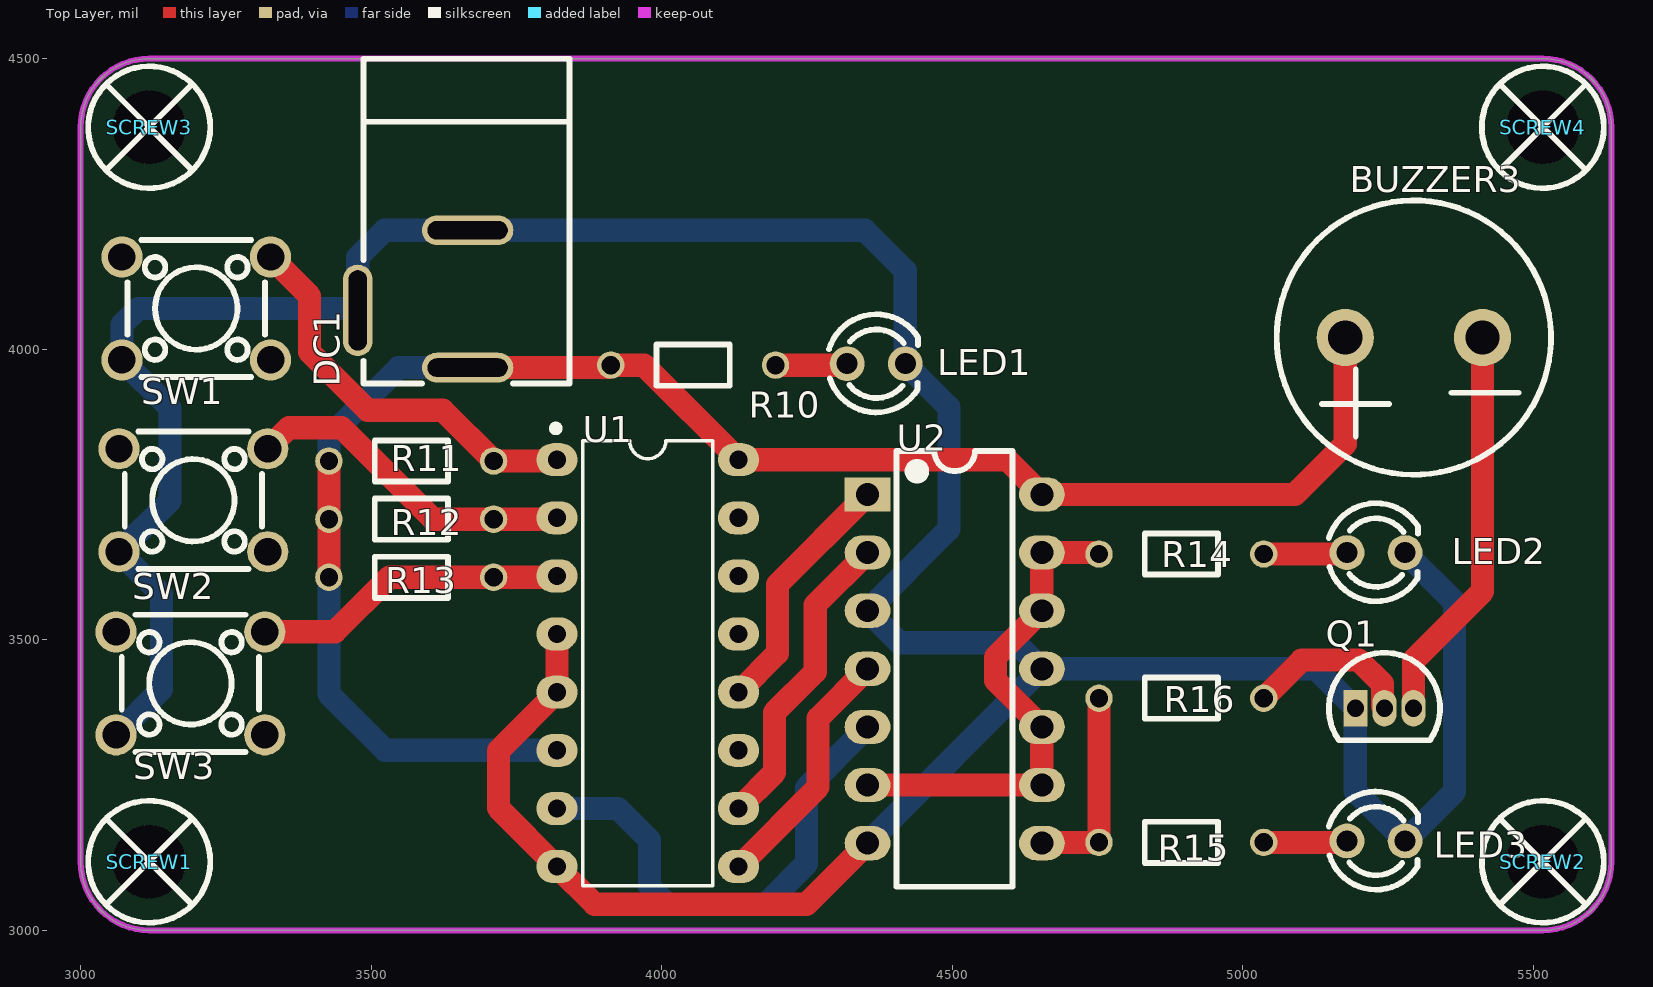
[diagram p0: Top Layer view]
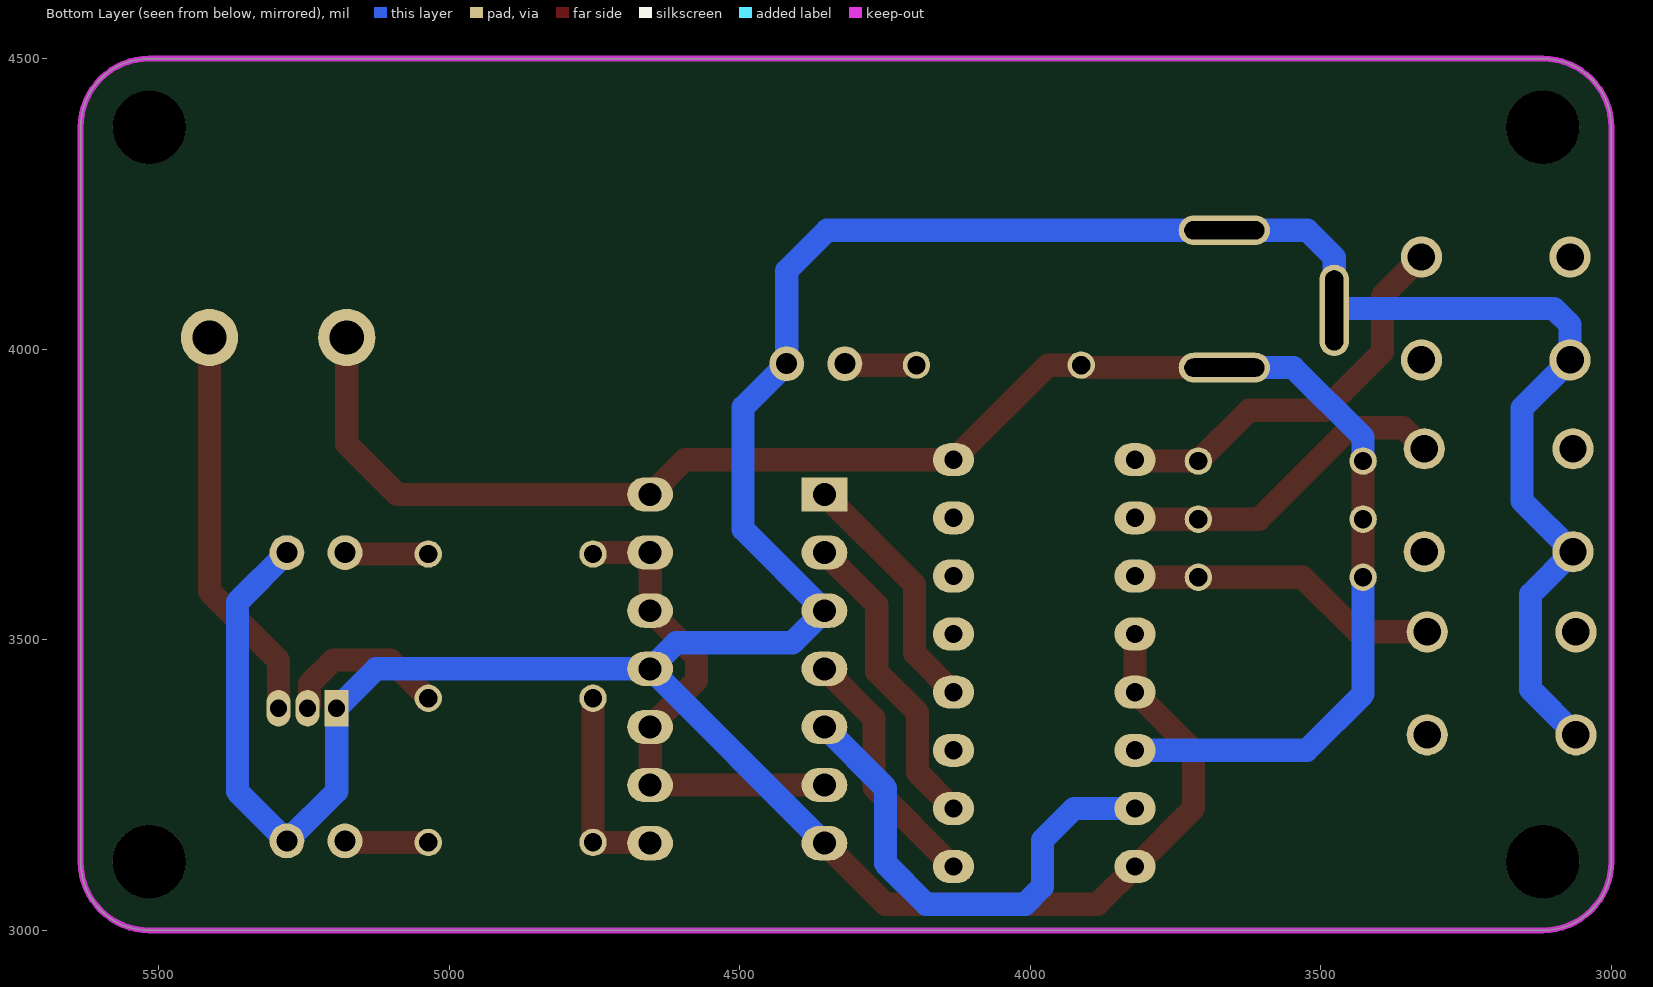
[diagram p1: Bottom Layer view, seen from below]
# Altium PCB MISC51615.pcbdoc
Units mil, origin at the board's own origin, x right, y up, seen from the top; angles counter-clockwise.
Board outline 2634 x 1500 mil, 2 copper layers (Top Layer, Bottom Layer), stack 62.206 mil thick; 22 components, 16 nets, 74 pads, 0 vias.

## Layer stack, top to bottom
Top Solder Mask Layer: solder mask 0.394, Dk 3.3
Top Layer: signal copper 1.379
Dielectric1: surface 59.449, FR4, Dk 4.5
Bottom Layer: signal copper 1.378
Bottom Solder Mask Layer: solder mask 0.394, Dk 3.3

## Board outline
3118.11,4500 ccw(c3118.11,4381.89) 3000,4381.89 3000,3118.11 ccw(c3118.11,3118.11) 3118.11,3000 5515.89,3000 ccw(c5515.89,3118.11) 5634,3118.11 5634,4381.89 ccw(c5515.89,4381.89) 5515.89,4500

## Design rules (kind name [scope] priority, off if disabled: settings)
BoardOutlineClearance copperThickness2oz_1 [All] p2 off: genericclearance=7.99 ignorepadtopadclearanceinfootprint=FALSE except(0: Arc-SplitContinuation Track-SplitContinuation SMDPad-SplitContinuation THPad-SplitContinuation Via-SplitContinuation Fill-SplitContinuation Region-SplitContinuation Poly-SplitContinuation Text-SplitContinuation Hole-SplitContinuation; 5.98: Arc-CutoutEdge Track-CutoutEdge SMDPad-CutoutEdge THPad-CutoutEdge Via-CutoutEdge Text-CutoutEdge; 6.9: Hole-OutlineEdge Hole-CutoutEdge; 10: Poly-OutlineEdge Poly-CutoutEdge; 11.81: Arc-OutlineEdge Track-OutlineEdge SMDPad-OutlineEdge THPad-OutlineEdge Via-OutlineEdge Fill-OutlineEdge Region-OutlineEdge Text-OutlineEdge Fill-CutoutEdge Region-CutoutEdge)
BoardOutlineClearance Plane_innerPlane_1 [All] p4 off: genericclearance=4.02 ignorepadtopadclearanceinfootprint=FALSE except(0: Arc-SplitContinuation Track-SplitContinuation SMDPad-SplitContinuation THPad-SplitContinuation Via-SplitContinuation Fill-SplitContinuation Region-SplitContinuation Poly-SplitContinuation Text-SplitContinuation Hole-SplitContinuation; 5.98: Arc-CutoutEdge Track-CutoutEdge SMDPad-CutoutEdge THPad-CutoutEdge Via-CutoutEdge Text-CutoutEdge; 6.9: Hole-OutlineEdge Hole-CutoutEdge; 10: Poly-OutlineEdge Poly-CutoutEdge; 11.81: Arc-OutlineEdge Track-OutlineEdge SMDPad-OutlineEdge THPad-OutlineEdge Via-OutlineEdge Fill-OutlineEdge Region-OutlineEdge Text-OutlineEdge Fill-CutoutEdge Region-CutoutEdge)
BoardOutlineClearance Copper_copperRegion_1 [All] p6 off: genericclearance=4.02 ignorepadtopadclearanceinfootprint=FALSE except(0: Arc-SplitContinuation Track-SplitContinuation SMDPad-SplitContinuation THPad-SplitContinuation Via-SplitContinuation Fill-SplitContinuation Region-SplitContinuation Poly-SplitContinuation Text-SplitContinuation Hole-SplitContinuation; 5.98: Arc-CutoutEdge Track-CutoutEdge SMDPad-CutoutEdge THPad-CutoutEdge Via-CutoutEdge Text-CutoutEdge; 6.9: Hole-OutlineEdge Hole-CutoutEdge; 10: Poly-OutlineEdge Poly-CutoutEdge; 11.81: Arc-OutlineEdge Track-OutlineEdge SMDPad-OutlineEdge THPad-OutlineEdge Via-OutlineEdge Fill-OutlineEdge Region-OutlineEdge Text-OutlineEdge Fill-CutoutEdge Region-CutoutEdge)
BoardOutlineClearance copperThickness1oz_1 [All] p8: genericclearance=4.02 ignorepadtopadclearanceinfootprint=FALSE except(0: Arc-SplitContinuation Track-SplitContinuation SMDPad-SplitContinuation THPad-SplitContinuation Via-SplitContinuation Fill-SplitContinuation Region-SplitContinuation Poly-SplitContinuation Text-SplitContinuation Hole-SplitContinuation; 5.98: Arc-CutoutEdge Track-CutoutEdge SMDPad-CutoutEdge THPad-CutoutEdge Via-CutoutEdge Text-CutoutEdge; 6.9: Hole-OutlineEdge Hole-CutoutEdge; 10: Poly-OutlineEdge Poly-CutoutEdge; 11.81: Arc-OutlineEdge Track-OutlineEdge SMDPad-OutlineEdge THPad-OutlineEdge Via-OutlineEdge Fill-OutlineEdge Region-OutlineEdge Text-OutlineEdge Fill-CutoutEdge Region-CutoutEdge)
Clearance copperThickness2oz [All] p1 off: gap=7.99 ignorepadtopadclearanceinfootprint=FALSE except(5.98: SMDPad-Track SMDPad-SMDPad THPad-Track SMDPad-THPad THPad-THPad Track-Via SMDPad-Via THPad-Via Via-Via Fill-SMDPad Region-SMDPad Fill-THPad Region-THPad Fill-Via Region-Via Fill-Fill Fill-Region Region-Region Arc-Track Arc-SMDPad Arc-THPad Arc-Via Fill-Arc Region-Arc Arc-Arc Text-Track SMDPad-Text Text-THPad Text-Via Fill-Text Region-Text Arc-Text Text-Text; 6.9: Hole-Track Hole-SMDPad Hole-THPad Hole-Via Fill-Hole Region-Hole Hole-Arc Hole-Text; 10: Poly-Track Poly-SMDPad Poly-THPad Poly-Via Poly-Fill Poly-Region Poly-Poly Poly-Arc Poly-Text Poly-Hole; 11.81: Fill-Track Region-Track)
Clearance Plane_innerPlane [All] p3 off: gap=4.02 ignorepadtopadclearanceinfootprint=FALSE except(5.98: SMDPad-Track SMDPad-SMDPad THPad-Track SMDPad-THPad THPad-THPad Track-Via SMDPad-Via THPad-Via Via-Via Fill-SMDPad Region-SMDPad Fill-THPad Region-THPad Fill-Via Region-Via Fill-Fill Fill-Region Region-Region Arc-Track Arc-SMDPad Arc-THPad Arc-Via Fill-Arc Region-Arc Arc-Arc Text-Track SMDPad-Text Text-THPad Text-Via Fill-Text Region-Text Arc-Text Text-Text; 6.9: Hole-Track Hole-SMDPad Hole-THPad Hole-Via Fill-Hole Region-Hole Hole-Arc Hole-Text; 10: Poly-Track Poly-SMDPad Poly-THPad Poly-Via Poly-Fill Poly-Region Poly-Poly Poly-Arc Poly-Text Poly-Hole; 11.81: Fill-Track Region-Track)
Clearance Copper_copperRegion [All] p5 off: gap=4.02 ignorepadtopadclearanceinfootprint=FALSE except(5.98: SMDPad-Track SMDPad-SMDPad THPad-Track SMDPad-THPad THPad-THPad Track-Via SMDPad-Via THPad-Via Via-Via Fill-SMDPad Region-SMDPad Fill-THPad Region-THPad Fill-Via Region-Via Fill-Fill Fill-Region Region-Region Arc-Track Arc-SMDPad Arc-THPad Arc-Via Fill-Arc Region-Arc Arc-Arc Text-Track SMDPad-Text Text-THPad Text-Via Fill-Text Region-Text Arc-Text Text-Text; 6.9: Hole-Track Hole-SMDPad Hole-THPad Hole-Via Fill-Hole Region-Hole Hole-Arc Hole-Text; 10: Poly-Track Poly-SMDPad Poly-THPad Poly-Via Poly-Fill Poly-Region Poly-Poly Poly-Arc Poly-Text Poly-Hole; 11.81: Fill-Track Region-Track)
Clearance copperThickness1oz [All] p7: gap=4.02 ignorepadtopadclearanceinfootprint=FALSE except(5.98: SMDPad-Track SMDPad-SMDPad THPad-Track SMDPad-THPad THPad-THPad Track-Via SMDPad-Via THPad-Via Via-Via Fill-SMDPad Region-SMDPad Fill-THPad Region-THPad Fill-Via Region-Via Fill-Fill Fill-Region Region-Region Arc-Track Arc-SMDPad Arc-THPad Arc-Via Fill-Arc Region-Arc Arc-Arc Text-Track SMDPad-Text Text-THPad Text-Via Fill-Text Region-Text Arc-Text Text-Text; 6.9: Hole-Track Hole-SMDPad Hole-THPad Hole-Via Fill-Hole Region-Hole Hole-Arc Hole-Text; 10: Poly-Track Poly-SMDPad Poly-THPad Poly-Via Poly-Fill Poly-Region Poly-Poly Poly-Arc Poly-Text Poly-Hole; 11.81: Fill-Track Region-Track)
DiffPairsRouting differentialPair [All] p1: maxlimit=6 minlimit=6 mostfreqgap=6 toplayer_minwidth=5 toplayer_prefwidth=10 toplayer_maxwidth=100 toplayer_mingap=6 toplayer_prefgap=6 toplayer_maxgap=6 bottomlayer_minwidth=5 bottomlayer_prefwidth=10 bottomlayer_maxwidth=100 bottomlayer_mingap=6 bottomlayer_prefgap=6 bottomlayer_maxgap=6 maxuncoupledlength=10
HoleToHoleClearance otherClearance [All] p1: gap=11.81 allowstackedmicrovias=TRUE
Length netLength [All] p1: minlimit=0 maxlimit=0
PasteMaskExpansion pasteMaskExpansion [All] p1: expansion=0
PlaneConnect innerPlane [All] p1: planeconnectstyle=Relief reliefexpansion=20 reliefentries=4 reliefconductorwidth=10 reliefairgap=10
PolygonConnect copperRegion [All] p1: connectstyle=Relief reliefconductorwidth=10 reliefentries=4 polygonreliefangle="90 Angle" airgapwidth=10 via.connectstyle=Relief via.reliefconductorwidth=10 via.reliefentries=4 via.polygonreliefangle="90 Angle" via.airgapwidth=10
RoutingVias viaSize [All] p1: holewidth=12.01 width=24.02 viastyle="Through Hole" minholewidth=11.81 minwidth=19.68 maxholewidth=248.03 maxwidth=393.7
SolderMaskExpansion solderMaskExpansion [IsVia] p1: expansion=-1000 istentingtop=TRUE
SolderMaskExpansion solderMaskExpansion [All] p2: expansion=2 istentingtop=FALSE
Width copperThickness2oz_2 [All] p1 off: maxlimit=100 minlimit=8 preferedwidth=10
Width copperThickness1oz_2 [All] p2: maxlimit=100 minlimit=5 preferedwidth=10

## Components (designator, comment, footprint, x,y, rotation, side; value= is the part's Value field where it differs from the comment)
BUZZER3 "buzzer" BUZ-TH_BD12.0-P6.00-D0.9-RD 5294.02,4020 r180 top
DC1 "" DC-2.0 3676.42,4091.4 r90 top
LED1 "" LED_TH-3mm 4369.02,3975 r0 top
LED2 "" LED_TH-3mm 5229.02,3650 r0 top
LED3 "" LED_TH-3mm 5229.02,3153.82 r0 top
Q1 "SS8050BBU" TO-92-3_L4.8-W3.7-P1.27-L-1 5243.41,3382.11 r0 top
R10 "1kΩ" Res_1/8W 4054.02,3975 r180 top
R11 "10kΩ" Res_1/8W 3569.02,3810 r180 top
R12 "10kΩ" Res_1/8W 3569.02,3710 r180 top
R13 "10kΩ" Res_1/8W 3569.02,3610 r180 top
R14 "510Ω" Res_1/8W 4894.02,3650 r180 top
R15 "510Ω" Res_1/8W 4894.02,3153.82 r180 top
R16 "10kΩ" Res_1/8W 4894.02,3396.95 r0 top
SCREW1 "" M3螺丝 3118.11,3118.11 r0 top
SCREW2 "" M3螺丝 5515.91,3118.11 r0 top
SCREW3 "" M3螺丝 3118.11,4381.89 r0 top
SCREW4 "" M3螺丝 5515.91,4381.89 r0 top
SW1 "" SW-TH_4P-L6.0-W6.0-P4.50-LS6.5 3199.02,4070 r180 top
SW2 "" SW-TH_4P-L6.0-W6.0-P4.50-LS6.5 3194.02,3740 r180 top
SW3 "" SW-TH_4P-L6.0-W6.0-P4.50-LS6.5 3189.02,3425 r180 top
U1 "SN74HC138N(LX)" PDIP-16_L19.3-W6.4-P2.54-LS7.94-BL 3975.87,3459.79 r270 top
U2 "SN74HC20N(LX)" PDIP-14_L19.3-W6.5-P2.54-LS7.6-BL 4504.02,3450 r270 top

## Footprints (in the part's own frame and the unit in brackets; to place one, negate y for a bottom-side part, rotate by r counter-clockwise, add the part's x,y. Pads: shape width x height; smd on the part's side, far side on the other; paste and mask are expansions set on the pad)
BUZ-TH_BD12.0-P6.00-D0.9-RD [mm]
  round 2.5 hole 1.5 paste+0 mask+0.05: 1(-3,0) 2(3,0)
  silkscreen extent -5.99,-5.99 5.99,5.99
DC-2.0 [mil]
  oval 157.5x51.2 hole 31.5 slot 137.8 at 0 deg paste+0 mask+2: 2(-24.7,199.5)
  oval 51.2x157.5 hole 31.5 slot 137.8 at 90 deg paste+0 mask+2: 3(113.1,10.5) 4(-123.1,10.5)
  silkscreen extent -151,-165 408,190
LED_TH-3mm [mil]
  round 60 hole 36 paste+0 mask+2: 1(-50,0) 2(50,0)
  silkscreen extent -81,-84 72,85
M3螺丝 [mil]
  round 126 hole 126 paste+0 mask+4: 1(0,0)
  silkscreen extent -105,-105 105,105
PDIP-14_L19.3-W6.5-P2.54-LS7.6-BL [mm]
  rect 1.5x2 hole 1: 1(-7.62,-3.81)
  oval 1.5x2 hole 1: 2(-5.08,-3.81) 3(-2.54,-3.81) 4(0,-3.81) 5(2.54,-3.81) 6(5.08,-3.81) 7(7.62,-3.81) 8(7.62,3.81) 9(5.08,3.81) 10(2.54,3.81) 11(0,3.81) 12(-2.54,3.81) 13(-5.08,3.81) 14(-7.62,3.81)
  silkscreen extent -9.53,-2.55 9.53,2.53
PDIP-16_L19.3-W6.4-P2.54-LS7.94-BL [mm]
  oval 1.44x1.8 hole 0.8: 1(-8.89,-3.97) 2(-6.35,-3.97) 3(-3.81,-3.97) 4(-1.27,-3.97) 5(1.27,-3.97) 6(3.81,-3.97) 7(6.35,-3.97) 8(8.89,-3.97) 9(8.89,3.97) 10(6.35,3.97) 11(3.81,3.97) 12(1.27,3.97) 13(-1.27,3.97) 14(-3.81,3.97) 15(-6.35,3.97) 16(-8.89,3.97)
  silkscreen extent -10.41,-4.17 9.73,2.84
Res_1/8W [mil]
  round 47.2 hole 31.5 paste+0 mask+2: 1(-141.7,2.48) 2(141.7,2.48)
  silkscreen extent -63,-33 63,38
SW-TH_4P-L6.0-W6.0-P4.50-LS6.5 [mm]
  round 1.8 hole 1.2: 1(-3.25,2.25) 2(3.25,2.25) 3(-3.25,-2.25) 4(3.25,-2.25)
  silkscreen extent -3,-3 3,3
TO-92-3_L4.8-W3.7-P1.27-L-1 [mm]
  rect 1.05x1.6 hole 0.75: 1(-1.27,0)
  oval 1.05x1.6 hole 0.75: 2(0,0) 3(1.27,0)
  silkscreen extent -2.43,-1.39 2.43,2.43

## Nets (pads, with @x,y where several pads share a name; then routed paths per layer and width w, separated by ;. In a path a pad name is that pad's centre, name@x,y a point inside that pad or via, vN(x,y) a via of type N, cw(c..) or ccw(c..) an arc to the next point about the centre after c; other vN are vias at no path point)
$1N4636: LED1.1 R10.1 | length 124.3
  Top Layer w40: R10.1 4316.54,3972.52 LED1.1
$1N7161: R11.1 SW1.3 U1.1 | length 695.5
  Top Layer w40: SW1.3 3394.02,4091.53 3394.02,3995 3494.02,3895 3623.24,3895 R11.1 3817.3,3807.52 U1.1
$1N7170: R12.1 SW2.3 U1.2 | length 578.9
  Top Layer w40: SW2.3 3358.39,3865 3449.02,3865 3606.5,3707.52 R12.1 3817.3,3707.52 U1.2
$1N7174: R13.1 SW3.3 U1.3 | length 542.5
  Top Layer w40: SW3.3 3437.6,3513.58 3531.54,3607.52 R13.1 3817.3,3607.52 U1.3
$1N7496: U1.12 U2.1 | length 432.1
  Top Layer w40: U1.12 4199.02,3476.64 4199.02,3595 U2.1
$1N7656: U1.10 U2.2 | length 532.1
  Top Layer w40: U1.10 4194.02,3271.64 4194.02,3375 4264.02,3445 4264.02,3560 U2.2
$1N7664: U1.9 U2.4 | length 432.1
  Top Layer w40: U1.9 4269.02,3246.64 4269.02,3365 U2.4
$1N7674: U1.7 U2.5 | length 852.1
  Bottom Layer w40: U1.7 3924.23,3209.79 3979.02,3155 3979.02,3075 4009.02,3045 4179.02,3045 4249.02,3115 4249.02,3245 U2.5
$1N7682: R14.2 U2.6 U2.9 U2.10 U2.12 U2.13 | length 865.6
  Top Layer w40: U2.6 U2.9 U2.10 4574.02,3430 4574.02,3470 U2.12 U2.13 4749.84,3650 R14.2
$1N7700: R15.2 R16.1 U2.8 | length 346.9
  Top Layer w40: U2.8 4655.36,3151.34 R15.2 R16.1
$1N7868: LED2.1 R14.1 | length 144.3
  Top Layer w40: R14.1 5176.54,3647.52 LED2.1
$1N7967: LED3.1 R15.1 | length 144.3
  Top Layer w40: R15.1 5176.54,3151.34 LED3.1
$1N8159: BUZZER3.1 Q1.3 | length 687.1
  Top Layer w40: Q1.3 5293.41,3464.39 5412.13,3583.11 BUZZER3.1
$1N8195: Q1.2 R16.2 | length 292
  Top Layer w40: R16.2 5101.29,3465 5199.43,3465 5240.06,3424.36 5240.06,3385.45 Q1.2
+5V: BUZZER3.2 DC1.4 R10.2 R11.2 R12.2 R13.2 U1.6 U1.16 U2.14 | length 2985.3
  Top Layer w40: R13.2 R12.2 R11.2 ; DC1.4 3908.1,3968.3 R10.2 3969.43,3972.52 U1.16 4594.23,3809.79 U2.14 5089.02,3750 5175.91,3836.89 BUZZER3.2
  Bottom Layer w40: R13.2 3427.32,3406.7 3524.23,3309.79 U1.6 ; R11.2 3427.32,3848.3 3547.32,3968.3 DC1.4
GND: DC1.2 DC1.3 LED1.2 LED2.2 LED3.2 Q1.1 SW1.2 SW2.2 SW3.2 U1.4 U1.5 U1.8 U2.3 U2.7 U2.11 | length 6261.6
  Top Layer w40: U1.5@3814.19,3415.17 3819.57,3420.55 U1.4 ; U1.5 3719.02,3309.24 3719.02,3210.34 U1.8 3884.36,3045 4249.02,3045 U2.7
  Bottom Layer w40: SW3.2 3139.02,3414.37 3139.02,3578.47 SW2.2 3154.02,3739.37 3154.02,3898.47 SW1.2 3071.07,4042.05 3099.02,4070 3473.62,4070 DC1.2 3476.92,4157.9 3523.52,4204.5 DC1.3 4349.52,4204.5 4419.02,4135 LED1.2 4494.02,3900 4494.02,3690 U2.3 4409.02,3495 4609.02,3495 U2.11 ; U2.7 U2.11 ; LED2.2 5364.02,3565 5364.02,3238.82 LED3.2 5193.41,3239.43 Q1.1 5125.51,3450 U2.11
pads on no net: SCREW1.1 SCREW2.1 SCREW3.1 SCREW4.1 SW1.1 SW1.4 SW2.1 SW2.4 SW3.1 SW3.4 U1.11 U1.13 U1.14 U1.15

## Keep-outs
Board Outline Layer:
  the board outline again, w10

## Silkscreen, mask and mechanical layers (free items; w line width, h text height)
Top Silkscreen Layer: